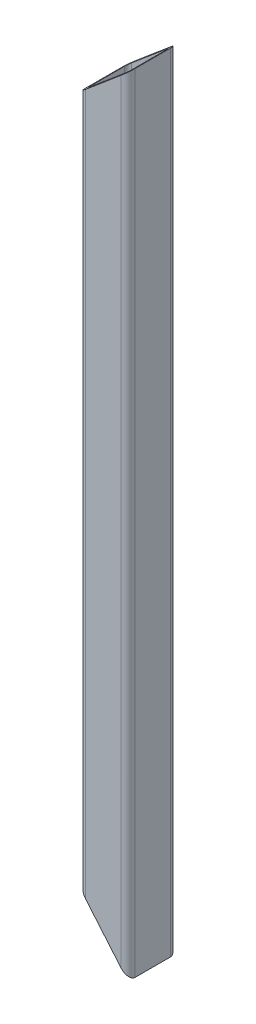
SolidWorks part; units mm, degrees
material "XRAAT"
ref_plane "前视基准面" through (0, 0, 0) normal (0, 0, 1) x (1, 0, 0)
ref_plane "上视基准面" through (0, 0, 0) normal (0, 1, 0) x (1, 0, 0)
ref_plane "右视基准面" through (0, 0, 0) normal (1, 0, 0) x (0, 0, -1)
sketch "草图1" plane through (0, 0, 0) normal (0, 0, 1) x (1, 0, 0)
  line L0 (0, 0) -> (0, 1116)
  dimension "D1" = 1116
other "结构用冷弯空心方钢(gb t6728-2002) 70×70×5(1)"
ref_plane "基准面1" through (0, 0, 0) normal (0, 1, 0) x (-1, 0, 0)
sketch "Sketch1" plane through (0, 0, 0) normal (0, 1, 0) x (-1, 0, 0)
  line L0 (-25, -30) -> (25, -30)
  line L1 (-30, -25) -> (-30, 25)
  line L2 (25, 30) -> (-25, 30)
  line L3 (30, 25) -> (30, -25)
  line L4 (-25, -35) -> (25, -35)
  line L5 (-35, -25) -> (-35, 25)
  line L6 (25, 35) -> (-25, 35)
  line L7 (35, 25) -> (35, -25)
  arc A0 (35, 25) -> (25, 35) centre (25, 25) ccw
  arc A1 (25, -35) -> (35, -25) centre (25, -25) ccw
  arc A2 (-35, -25) -> (-25, -35) centre (-25, -25) ccw
  arc A3 (-25, 35) -> (-35, 25) centre (-25, 25) ccw
  arc A4 (-25, 30) -> (-30, 25) centre (-25, 25) ccw
  arc A5 (30, 25) -> (25, 30) centre (25, 25) ccw
  arc A6 (25, -30) -> (30, -25) centre (25, -25) ccw
  arc A7 (-30, -25) -> (-25, -30) centre (-25, -25) ccw
  point P0 (-35, 0)
  point P1 (35, 0)
  point P2 (0, 35)
  point P3 (0, -35)
  point P4 (0, 0)
  point P5 (-35, -35)
  point P6 (35, -35)
  point P7 (35, 35)
  point P8 (-35, 35)
  point P33 (0, 0)
  dimension "D1" = 10
  dimension "D2" = 70
  dimension "D3" = 5
sketch "草图2" plane through (0, 0, 35) normal (0, 0, 1) x (1, 0, 0)
  line L0 (35, 1116) -> (-35, 1056.9639)
  line L1 (-35, 1116) -> (-35, 0) construction
  line L2 (-35, 1056.9639) -> (-35, 1116)
  line L3 (-35, 1116) -> (35, 1116)
  line L4 (-35, 83) -> (35, 0)
  line L5 (35, 0) -> (-35, 0)
  line L6 (-35, 0) -> (-35, 83)
  dimension "D1" = 83
  dimension "D2" = 90
  dimension "D3" = 59.0361
extrude "切除-拉伸1" cut sketch "草图2" against normal through all both and the other way through all
